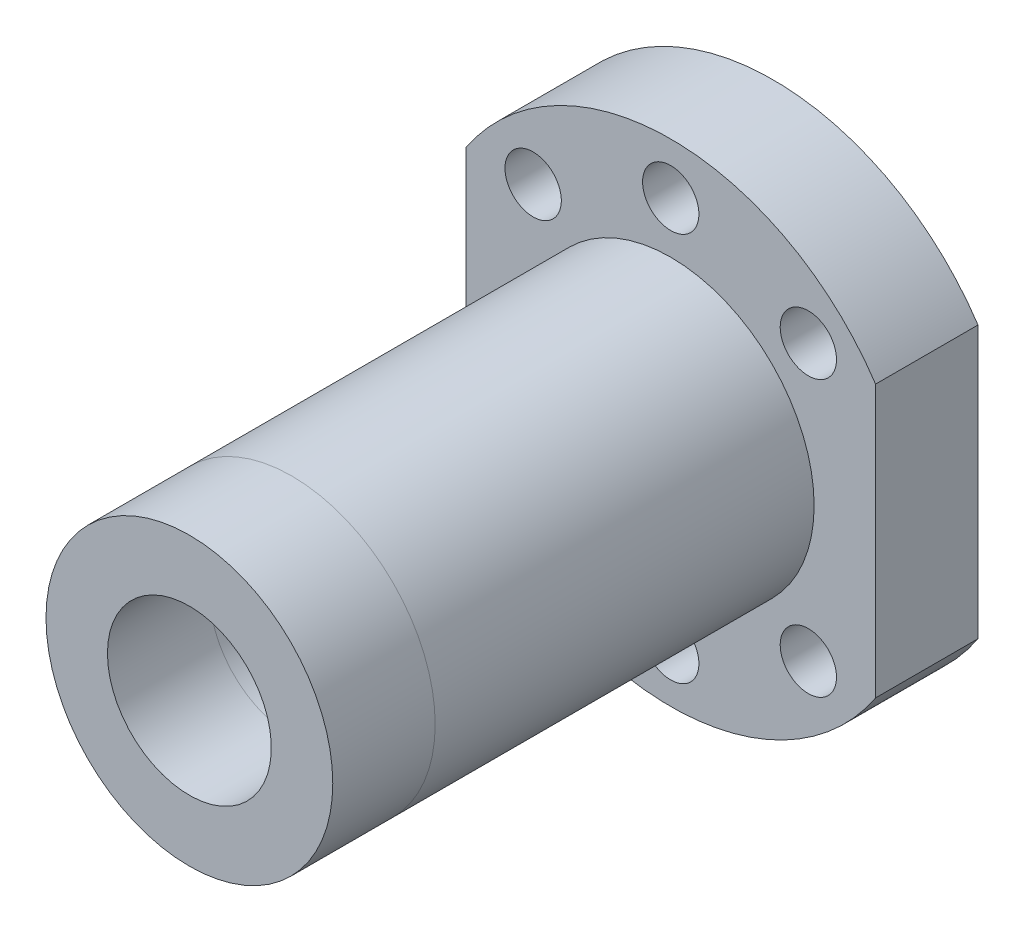
from build123d import *

# Parameters (mm, degrees)
SKETCH1_R                  = 14
SKETCH1_R_2                = 8
BOSS_EXTRUDE1_DEPTH        = 57
SKETCH2_R                  = 14
SKETCH2_R_2                = 8
BOSS_EXTRUDE2_DEPTH        = 10
F_5_5_5_5_DIAMETER_HOLE1_D = 5.5
SPLIT1_SURFACE_1_BACK      = 85.575
SPLIT1_SURFACE_1_DEPTH     = 171.15
SPLIT1_SURFACE_2_BACK      = 85.575
SPLIT1_SURFACE_2_DEPTH     = 171.15


with BuildPart() as part:
    # Sketch1 → Boss-Extrude1 (new body)
    with BuildSketch(Plane.XY):
        with Locations(Location((0, 0, 0), (0, 0, 180))):
            Circle(SKETCH1_R)
        with Locations(Location((0, 0, 0), (0, 0, 180))):
            Circle(SKETCH1_R_2, mode=Mode.SUBTRACT)
    extrude(amount=BOSS_EXTRUDE1_DEPTH)

    # Sketch2 → Boss-Extrude2 (add)
    # profile 1 of 2: a face of its own
    with BuildSketch(Plane(origin=(0, 0, 0), x_dir=(-1, 0, 0), z_dir=(0, 0, -1))):
        with BuildLine():
            ThreePointArc((20, 13.266499161), (0, 24), (-20, 13.266499161))
            Line((-20, 13.266499161), (-20, -13.266499161))
            ThreePointArc((-20, -13.266499161), (0, -24), (20, -13.266499161))
            Line((20, -13.266499161), (20, 13.266499161))
        make_face()
        Circle(SKETCH2_R, mode=Mode.SUBTRACT)
    # profile 2 of 2: a face of its own
    with BuildSketch(Plane(origin=(0, 0, 0), x_dir=(-1, 0, 0), z_dir=(0, 0, -1))):
        Circle(SKETCH2_R)
        Circle(SKETCH2_R_2, mode=Mode.SUBTRACT)
    extrude(amount=-BOSS_EXTRUDE2_DEPTH)

    # Ø5.5 (5.5) Diameter Hole1 (through all)
    with Locations(Plane(origin=(0, 0, 0), x_dir=(-1, 0, 0), z_dir=(0, 0, -1))):
        with Locations((0, 19), (-13.435028843, 13.435028843), (13.435028843, 13.435028843)):
            f_5_5_5_5_diameter_hole1 = Hole(F_5_5_5_5_DIAMETER_HOLE1_D / 2)

    # Mirror1: Ø5.5 (5.5) Diameter Hole1 across plane
    add(f_5_5_5_5_diameter_hole1.mirror(Plane.ZX), mode=Mode.SUBTRACT)


with BuildPart() as body_2:
    # Split1: the piece behind the surface
    add(part.part)
    # Split1 surface: a surface, the sketch's curves swept straight by 171.15 mm
    with BuildLine(Plane(origin=(0, 0, 0), x_dir=(1, 0, 0), z_dir=(0, 1, 0)).offset(-SPLIT1_SURFACE_1_BACK), mode=Mode.PRIVATE) as split1_surface_1_path:
        Line((-26.149288563, -10), (31.044229279, -10))
        Line((31.044229279, -10), (31.044229279, -47))
        Line((31.044229279, -47), (-26.149288563, -47))
        Line((-26.149288563, -47), (-26.149288563, -10))
    split1_surface_1 = Shell.extrude(split1_surface_1_path.wire(), (0 * SPLIT1_SURFACE_1_DEPTH, 1 * SPLIT1_SURFACE_1_DEPTH, 0 * SPLIT1_SURFACE_1_DEPTH))
    split(bisect_by=split1_surface_1, keep=Keep.BOTTOM)


with BuildPart() as part_1:
    add(part.part)

    # Split1: split by a surface, the side it looks to stays
    # Split1 surface: a surface, the sketch's curves swept straight by 171.15 mm
    with BuildLine(Plane(origin=(0, 0, 0), x_dir=(1, 0, 0), z_dir=(0, 1, 0)).offset(-SPLIT1_SURFACE_2_BACK), mode=Mode.PRIVATE) as split1_surface_2_path:
        Line((-26.149288563, -10), (31.044229279, -10))
        Line((31.044229279, -10), (31.044229279, -47))
        Line((31.044229279, -47), (-26.149288563, -47))
        Line((-26.149288563, -47), (-26.149288563, -10))
    split1_surface_2 = Shell.extrude(split1_surface_2_path.wire(), (0 * SPLIT1_SURFACE_2_DEPTH, 1 * SPLIT1_SURFACE_2_DEPTH, 0 * SPLIT1_SURFACE_2_DEPTH))
    split(bisect_by=split1_surface_2, keep=Keep.TOP)


solid = Compound([body_2.part, part_1.part])
